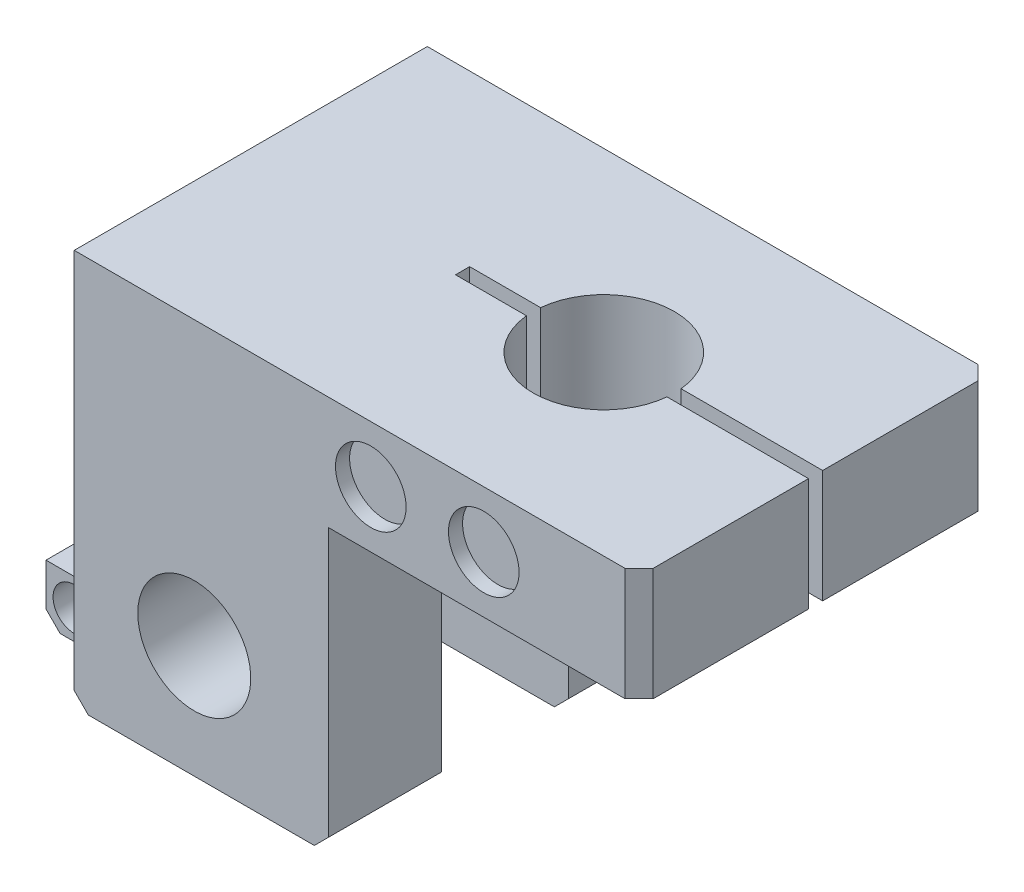
from build123d import *

# Parameters (mm, degrees)
SKETCH1_W           = 40
SKETCH1_H           = 25
BOSS_EXTRUDE1_DEPTH = 8
SKETCH3_R           = 5
CUT_EXTRUDE1_DEPTH  = 48.843494856
SKETCH4_W           = 25
SKETCH4_H           = 1
CUT_EXTRUDE2_DEPTH  = 48.843494856
SKETCH7_W           = 18
SKETCH7_H           = 8
BOSS_EXTRUDE2_DEPTH = 20
CHAMFER2_SIZE       = 1
SKETCH8_R           = 4
CUT_EXTRUDE3_DEPTH  = 52.23475383
SKETCH9_R           = 2.5
CUT_EXTRUDE4_DEPTH  = 1
CUT_EXTRUDE5_START  = -1
SKETCH10_R          = 2.5
CUT_EXTRUDE5_DEPTH  = 1
SKETCH11_W          = 4
SKETCH11_H          = 4
BOSS_EXTRUDE3_DEPTH = 6
SKETCH12_R          = 1.5
CUT_EXTRUDE6_DEPTH  = 20
CHAMFER4_SIZE       = 1


with BuildPart() as part:
    # Sketch1 → Boss-Extrude1 (new body)
    with BuildSketch(Plane(origin=(0, 0, 0), x_dir=(1, 0, 0), z_dir=(0, 1, 0))):
        with Locations((20, -12.5)):
            Rectangle(SKETCH1_W, SKETCH1_H)
    extrude(amount=BOSS_EXTRUDE1_DEPTH)

    # Sketch3 → Cut-Extrude1 (cut, through all)
    with BuildSketch(Plane(origin=(0, 8, 0), x_dir=(1, 0, 0), z_dir=(0, 1, 0))):
        with Locations(Location((25, -12.5, 0), (0, 0, 270))):
            Circle(SKETCH3_R)
    extrude(amount=-CUT_EXTRUDE1_DEPTH, mode=Mode.SUBTRACT)

    # Sketch4 → Cut-Extrude2 (cut, through all)
    with BuildSketch(Plane(origin=(0, 8, 0), x_dir=(1, 0, 0), z_dir=(0, 1, 0))):
        with Locations((27.5, -12.5)):
            Rectangle(SKETCH4_W, SKETCH4_H)
    extrude(amount=-CUT_EXTRUDE2_DEPTH, mode=Mode.SUBTRACT)

    # Sketch7 → Boss-Extrude2 (add)
    with BuildSketch(Plane.XZ):
        with Locations((9, 4)):
            Rectangle(SKETCH7_W, SKETCH7_H)
        with Locations((9, 21)):
            Rectangle(SKETCH7_W, SKETCH7_H)
    extrude(amount=BOSS_EXTRUDE2_DEPTH)

    # Chamfer2
    chamfer2_edges = [part.edges().sort_by_distance(p)[0] for p in [
        (18, -20, 4),
        (18, -20, 21),
        (40, 4, 0),
        (40, 4, 25),
    ]]
    chamfer(chamfer2_edges, length=CHAMFER2_SIZE)

    # Sketch8 → Cut-Extrude3 (cut, through all)
    with BuildSketch(Plane(origin=(0, 0, 0), x_dir=(-1, 0, 0), z_dir=(0, 0, -1))):
        with Locations((-8.5, -12)):
            Circle(SKETCH8_R)
    extrude(amount=-CUT_EXTRUDE3_DEPTH, mode=Mode.SUBTRACT)

    # Sketch9 → Cut-Extrude4 (cut)
    with BuildSketch(Plane(origin=(0, 0, 0), x_dir=(-1, 0, 0), z_dir=(0, 0, -1))):
        with Locations((-29, 4)):
            Circle(SKETCH9_R)
        with Locations((-21, 4)):
            Circle(SKETCH9_R)
    extrude(amount=-CUT_EXTRUDE4_DEPTH, mode=Mode.SUBTRACT)

    # Sketch10 → Cut-Extrude5 (cut)
    with BuildSketch(Plane.XY.offset(25).offset(CUT_EXTRUDE5_START)):
        with Locations(Location((21, 4, 0), (0, 0, 180))):
            Circle(SKETCH10_R)
        with Locations(Location((29, 4, 0), (0, 0, 180))):
            Circle(SKETCH10_R)
    extrude(amount=CUT_EXTRUDE5_DEPTH, mode=Mode.SUBTRACT)

    # Sketch11 → Boss-Extrude3 (add)
    with BuildSketch(Plane.ZY):
        with Locations((19, -18)):
            Rectangle(SKETCH11_W, SKETCH11_H)
        with Locations((6, -18)):
            Rectangle(SKETCH11_W, SKETCH11_H)
    extrude(amount=BOSS_EXTRUDE3_DEPTH)

    # Sketch12 → Cut-Extrude6 (cut)
    with BuildSketch(Plane(origin=(0, 0, 4), x_dir=(-1, 0, 0), z_dir=(0, 0, -1))):
        with Locations((4, -18)):
            Circle(SKETCH12_R)
    extrude(amount=-CUT_EXTRUDE6_DEPTH, mode=Mode.SUBTRACT)

    # Chamfer4
    chamfer4_edges = [part.edges().sort_by_distance(p)[0] for p in [
        (0, -20, 2),
        (-6, -20, 6),
        (-6, -20, 19),
        (0, -20, 23),
    ]]
    chamfer(chamfer4_edges, length=CHAMFER4_SIZE)


solid = part.part
